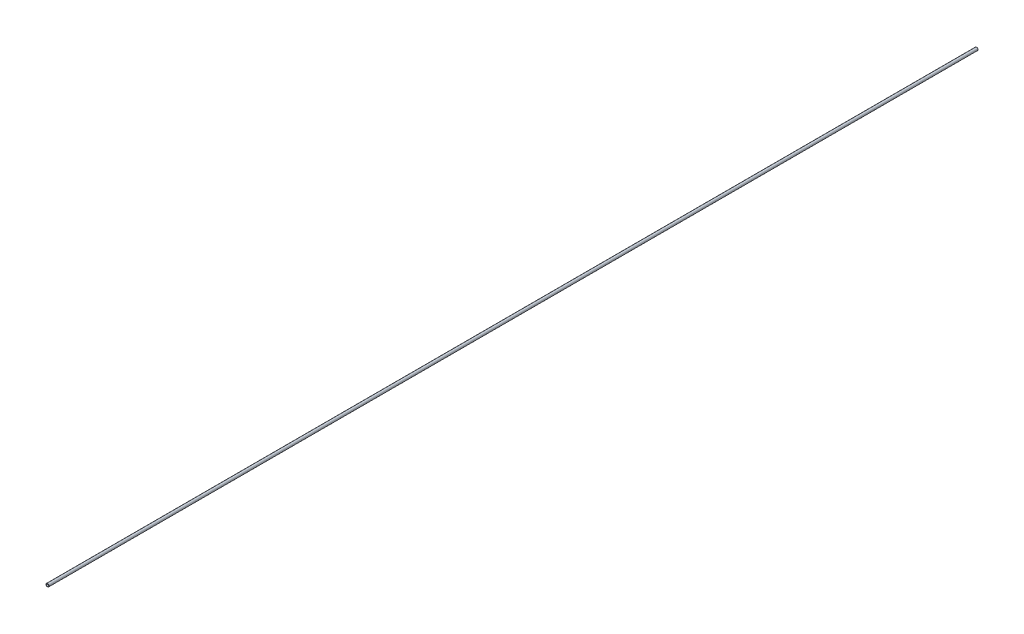
from build123d import *

# Parameters (mm, degrees)
SKETCH1_R           = 3
SKETCH1_R_2         = 2.25
BOSS_EXTRUDE1_DEPTH = 1900


with BuildPart() as part:
    # Sketch1 → Boss-Extrude1 (new body)
    with BuildSketch(Plane.XY):
        with Locations(Location((0, 0, 0), (0, 0, 180))):
            Circle(SKETCH1_R)
        with Locations(Location((0, 0, 0), (0, 0, 180))):
            Circle(SKETCH1_R_2, mode=Mode.SUBTRACT)
    extrude(amount=BOSS_EXTRUDE1_DEPTH)


solid = part.part
